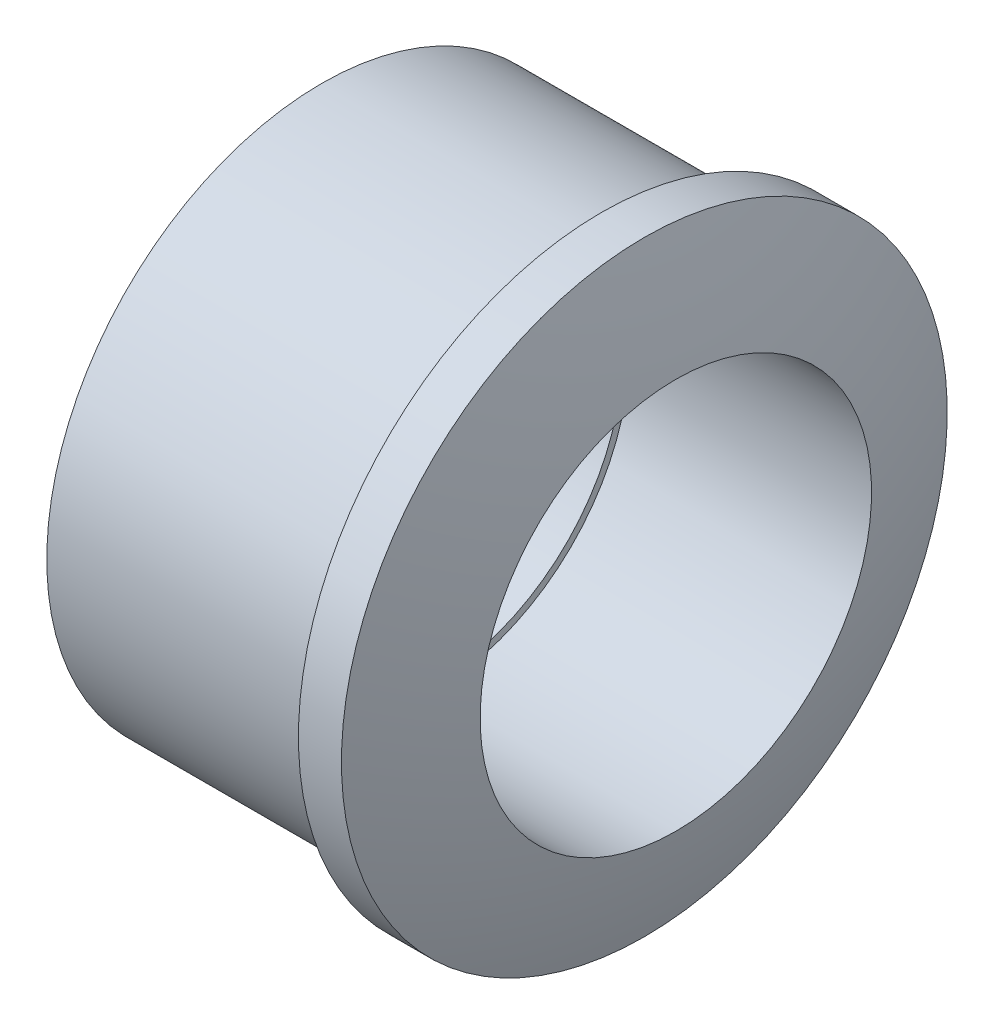
SolidWorks part; units mm, degrees
ref_plane "Front Plane" through (0, 0, 0) normal (0, 0, 1) x (1, 0, 0)
ref_plane "Top Plane" through (0, 0, 0) normal (0, 1, 0) x (1, 0, 0)
ref_plane "Right Plane" through (0, 0, 0) normal (1, 0, 0) x (0, 0, -1)
sketch "Sketch1" plane through (0, 0, 0) normal (0, 0, 1) x (1, 0, 0)
  line L0 (0, 0) -> (0, 29.5)
  line L1 (0, 29.5) -> (30, 29.5)
  line L2 (30, 29.5) -> (30, 32.5)
  line L3 (30, 32.5) -> (34.618, 32.5)
  line L4 (38, 21) -> (38, 0)
  line L5 (38, 0) -> (0, 0)
  arc A0 (34.618, 32.5) -> (38, 21) centre (-54.6499, 0) cw
  dimension "D3" = 95
  dimension "D1" = 29.5
  dimension "D2" = 30
  dimension "D4" = 21
  dimension "D5" = 38
  dimension "D6" = 32.5
revolve "Revolve1" add sketch "Sketch1" angle 360 about L5
sketch "Sketch3" plane through (0, 0, 0) normal (-1, 0, 0) x (0, 0, 1)
  circle A0 centre (0, 0) radius 20.25
  dimension "D1" = 40.5
extrude "Cut-Extrude2" cut sketch "Sketch3" against normal blind 12 separate body
sketch "Sketch2" plane through (0, 0, 0) normal (-1, 0, 0) x (0, 0, 1)
  circle A1 centre (0, 0) radius 29.5
  circle A2 centre (0, 0) radius 29.5
  dimension "D1" = 0
extrude "Cut-Extrude1" cut sketch "Sketch2" against normal blind 10 draft 75 separate body
sketch "Sketch4" plane through (12, 0, 0) normal (-1, 0, 0) x (0, 0, 1)
  circle A0 centre (0, 0) radius 21
  dimension "D1" = 42
extrude "Cut-Extrude3" cut sketch "Sketch4" against normal through all separate body
